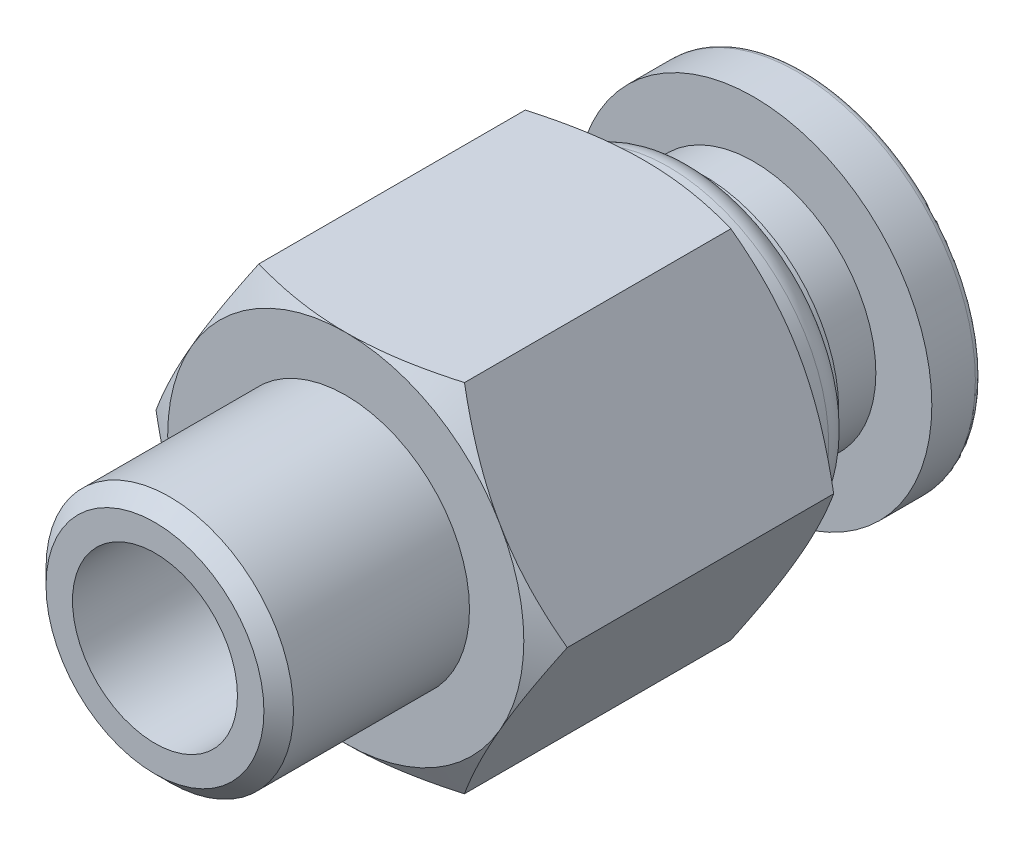
SolidWorks part; units mm, degrees
material "6061 合金"
ref_plane "前视基准面" through (0, 0, 0) normal (0, 0, 1) x (1, 0, 0)
ref_plane "上视基准面" through (0, 0, 0) normal (0, 1, 0) x (1, 0, 0)
ref_plane "右视基准面" through (0, 0, 0) normal (1, 0, 0) x (0, 0, -1)
sketch "草图1" plane through (0, 0, 0) normal (1, 0, 0) x (0, 0, -1)
  line L0 (-25.5, 3.2427) -> (-17, 3.2427)
  line L1 (-17, 3.2427) -> (-17, 4)
  line L2 (-17, 4) -> (0, 4)
  line L3 (0, 4) -> (0, 6.75)
  line L4 (-0.25, 7) -> (-1.9615, 7)
  line L5 (-1.9615, 7) -> (-1.9615, 4.8)
  line L6 (-1.9615, 4.8) -> (-3.9231, 4.8)
  line L7 (-3.9231, 4.8) -> (-3.9231, 5.3)
  line L8 (-3.9231, 5.3) -> (-4.3154, 5.3)
  line L9 (-5.3154, 6.3) -> (-6.2769, 6.3)
  line L10 (-6.2769, 6.3) -> (-6.2769, 7)
  line L11 (-6.2769, 7) -> (-6.9021, 8.0829)
  line L12 (-6.9021, 8.0829) -> (-17.3748, 8.0829)
  line L13 (-17.3748, 8.0829) -> (-18, 7)
  line L14 (-18, 7) -> (-18, 4.864)
  line L15 (-18, 4.864) -> (-24.919, 4.864)
  line L16 (-24.919, 4.864) -> (-25.5, 4.283)
  line L17 (-25.5, 4.283) -> (-25.5, 3.2427)
  line L18 (0, 0) -> (-25.5, 0) construction
  arc A0 (0, 6.75) -> (-0.25, 7) centre (-0.25, 6.75) ccw
  arc A1 (-4.3154, 5.3) -> (-5.3154, 6.3) centre (-5.3154, 5.3) ccw
revolve "旋转1" add sketch "草图1" angle 360 about L18
cosmetic thread "装饰螺纹线1" parameters "D1"=7.5, "D2"=8.566
ref_plane "基准面1" through (0, 0, 6.2769) normal (0, 0, -1) x (-1, 0, 0)
sketch "草图2" plane through (0, 0, 6.2769) normal (0, 0, -1) x (-1, 0, 0)
  line L0 (-4.0415, -7) -> (4.0415, -7)
  line L1 (4.0415, -7) -> (8.0829, 0)
  line L2 (8.0829, 0) -> (4.0415, 7)
  line L3 (4.0415, 7) -> (-4.0415, 7)
  line L4 (-4.0415, 7) -> (-8.0829, 0)
  line L5 (-8.0829, 0) -> (-4.0415, -7)
  circle A0 centre (0, 0) radius 14
extrude "切除-拉伸1" cut sketch "草图2" against normal blind 25.5
